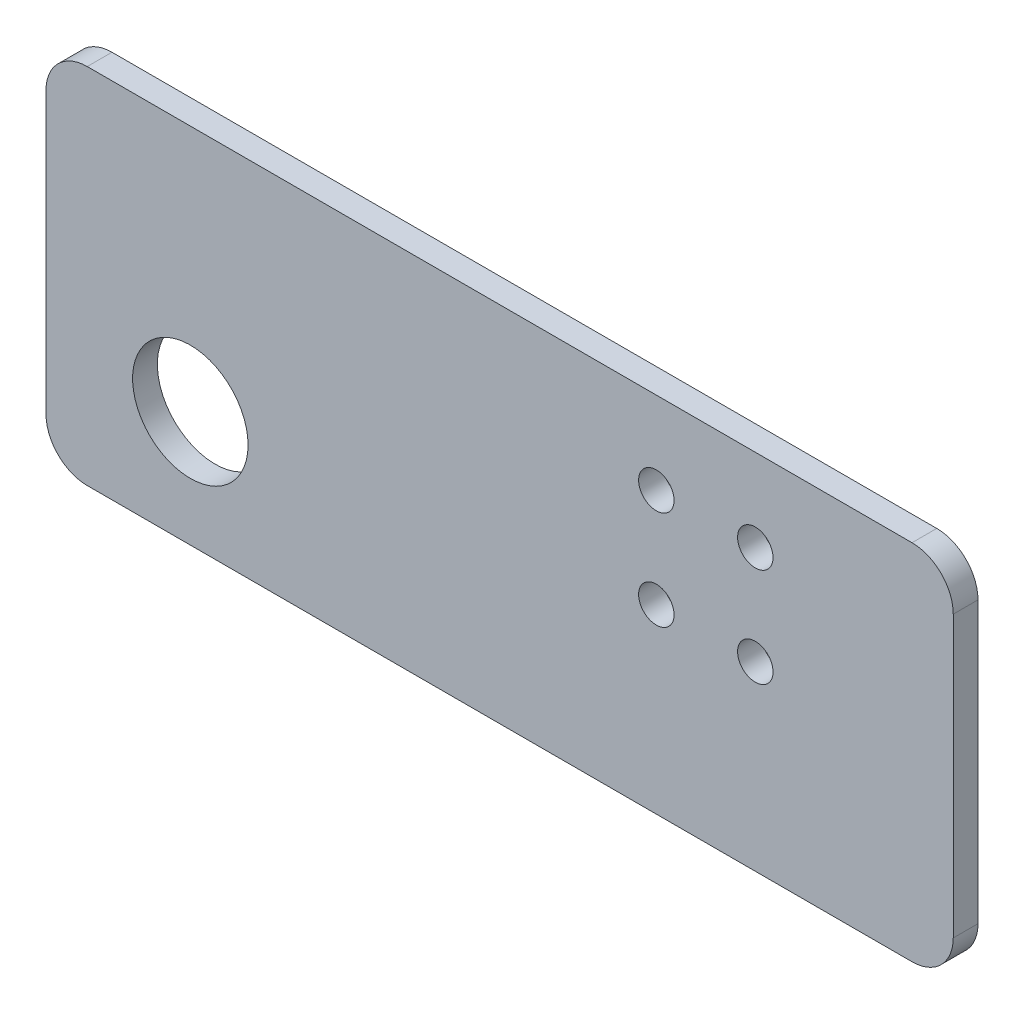
from build123d import *

# Parameters (mm, degrees)
SKETCH_1_W          = 160
SKETCH_1_H          = 44
EXTRUDE_1_DEPTH     = 3
SKETCH_2_R          = 7
SKETCH_2_R_2        = 2.15
CUT_EXTRUDE_1_DEPTH = 3
FILLET_1_R          = 5
SKETCH_3_W          = 63.678392254
SKETCH_3_H          = 72.512670224
CUT_EXTRUDE_2_DEPTH = 10
FILLET_2_R          = 5


with BuildPart() as part:
    # 草图1 → 凸台-拉伸1 (new body)
    with BuildSketch(Plane.XY):
        Rectangle(SKETCH_1_W, SKETCH_1_H)
    extrude(amount=EXTRUDE_1_DEPTH)

    # 草图2 → 切除-拉伸1 (cut)
    with BuildSketch(Plane.XY.offset(3)):
        with Locations((-62.5, -8)):
            Circle(SKETCH_2_R)
        with Locations((62.5, -8)):
            Circle(SKETCH_2_R)
        with Locations((-6, 12)):
            Circle(SKETCH_2_R_2)
        with Locations((6, 12)):
            Circle(SKETCH_2_R_2)
        with Locations((6, 0)):
            Circle(SKETCH_2_R_2)
        with Locations((-6, 0)):
            Circle(SKETCH_2_R_2)
    extrude(amount=-CUT_EXTRUDE_1_DEPTH, mode=Mode.SUBTRACT)

    # 圆角1
    fillet_1_edges = [part.edges().sort_by_distance(p)[0] for p in [
        (80, -22, 1.5),
        (-80, -22, 1.5),
        (-80, 22, 1.5),
        (80, 22, 1.5),
    ]]
    fillet(fillet_1_edges, radius=FILLET_1_R)

    # 草图3 → 切除-拉伸2 (cut)
    with BuildSketch(Plane.XY.offset(3)):
        with Locations((61.839196127, 0.092590352)):
            Rectangle(SKETCH_3_W, SKETCH_3_H)
    extrude(amount=-CUT_EXTRUDE_2_DEPTH, mode=Mode.SUBTRACT)

    # 圆角2
    fillet_2_edges = [part.edges().sort_by_distance(p)[0] for p in [
        (30, 22, 1.5),
        (30, -22, 1.5),
    ]]
    fillet(fillet_2_edges, radius=FILLET_2_R)


solid = part.part
